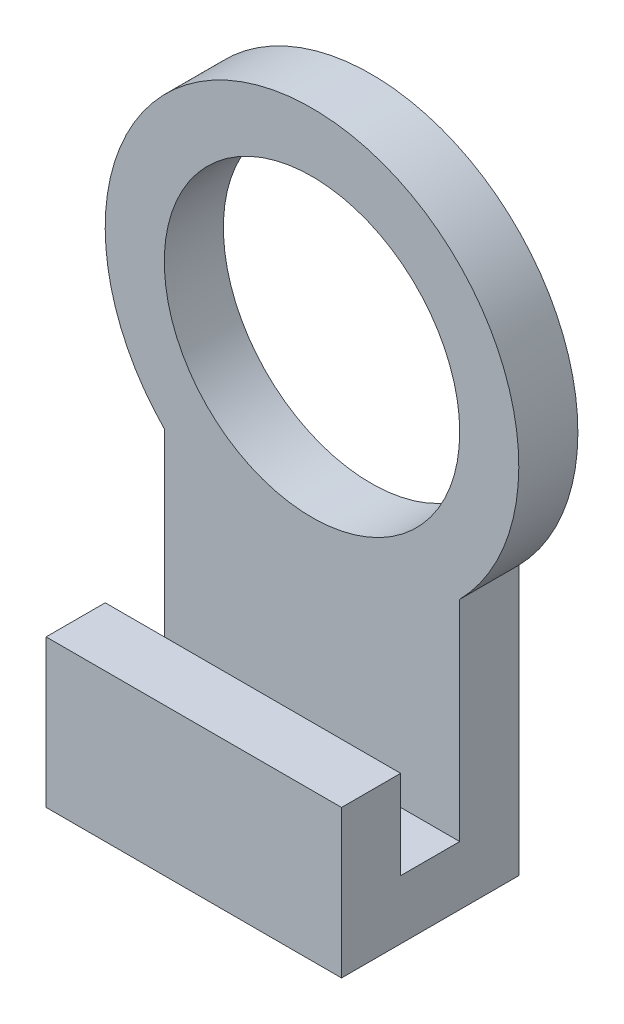
from build123d import *

# Parameters (mm, degrees)
BOSS_EXTRUDE1_DEPTH        = 4
SKETCH2_W                  = 20
SKETCH2_H                  = 4
BOSS_EXTRUDE2_DEPTH        = 8
SKETCH3_W                  = 20
SKETCH3_H                  = 4
BOSS_EXTRUDE3_DEPTH        = 6
F_20_0_20_DIAMETER_HOLE1_D = 20


with BuildPart() as part:
    # Sketch1 → Boss-Extrude1 (new body)
    with BuildSketch(Plane(origin=(0, 0, 0), x_dir=(-1, 0, 0), z_dir=(0, 0, -1))):
        with BuildLine():
            Line((-10, -28), (10, -28))
            Line((10, -28), (10, -9.797958971))
            ThreePointArc((10, -9.797958971), (0, 14), (-10, -9.797958971))
            Line((-10, -9.797958971), (-10, -28))
        make_face()
    extrude(amount=-BOSS_EXTRUDE1_DEPTH)

    # Sketch2 → Boss-Extrude2 (add)
    with BuildSketch(Plane.XY.offset(4)):
        with Locations((0, -26)):
            Rectangle(SKETCH2_W, SKETCH2_H)
    extrude(amount=BOSS_EXTRUDE2_DEPTH)

    # Sketch3 → Boss-Extrude3 (add)
    with BuildSketch(Plane(origin=(0, -24, 0), x_dir=(-1, 0, 0), z_dir=(0, 1, 0))):
        with Locations((0, 10)):
            Rectangle(SKETCH3_W, SKETCH3_H)
    extrude(amount=BOSS_EXTRUDE3_DEPTH)

    # Ø20.0 (20) Diameter Hole1 (through all)
    with Locations(Plane.XY.offset(4)):
        with Locations((0, 0)):
            Hole(F_20_0_20_DIAMETER_HOLE1_D / 2)


solid = part.part
